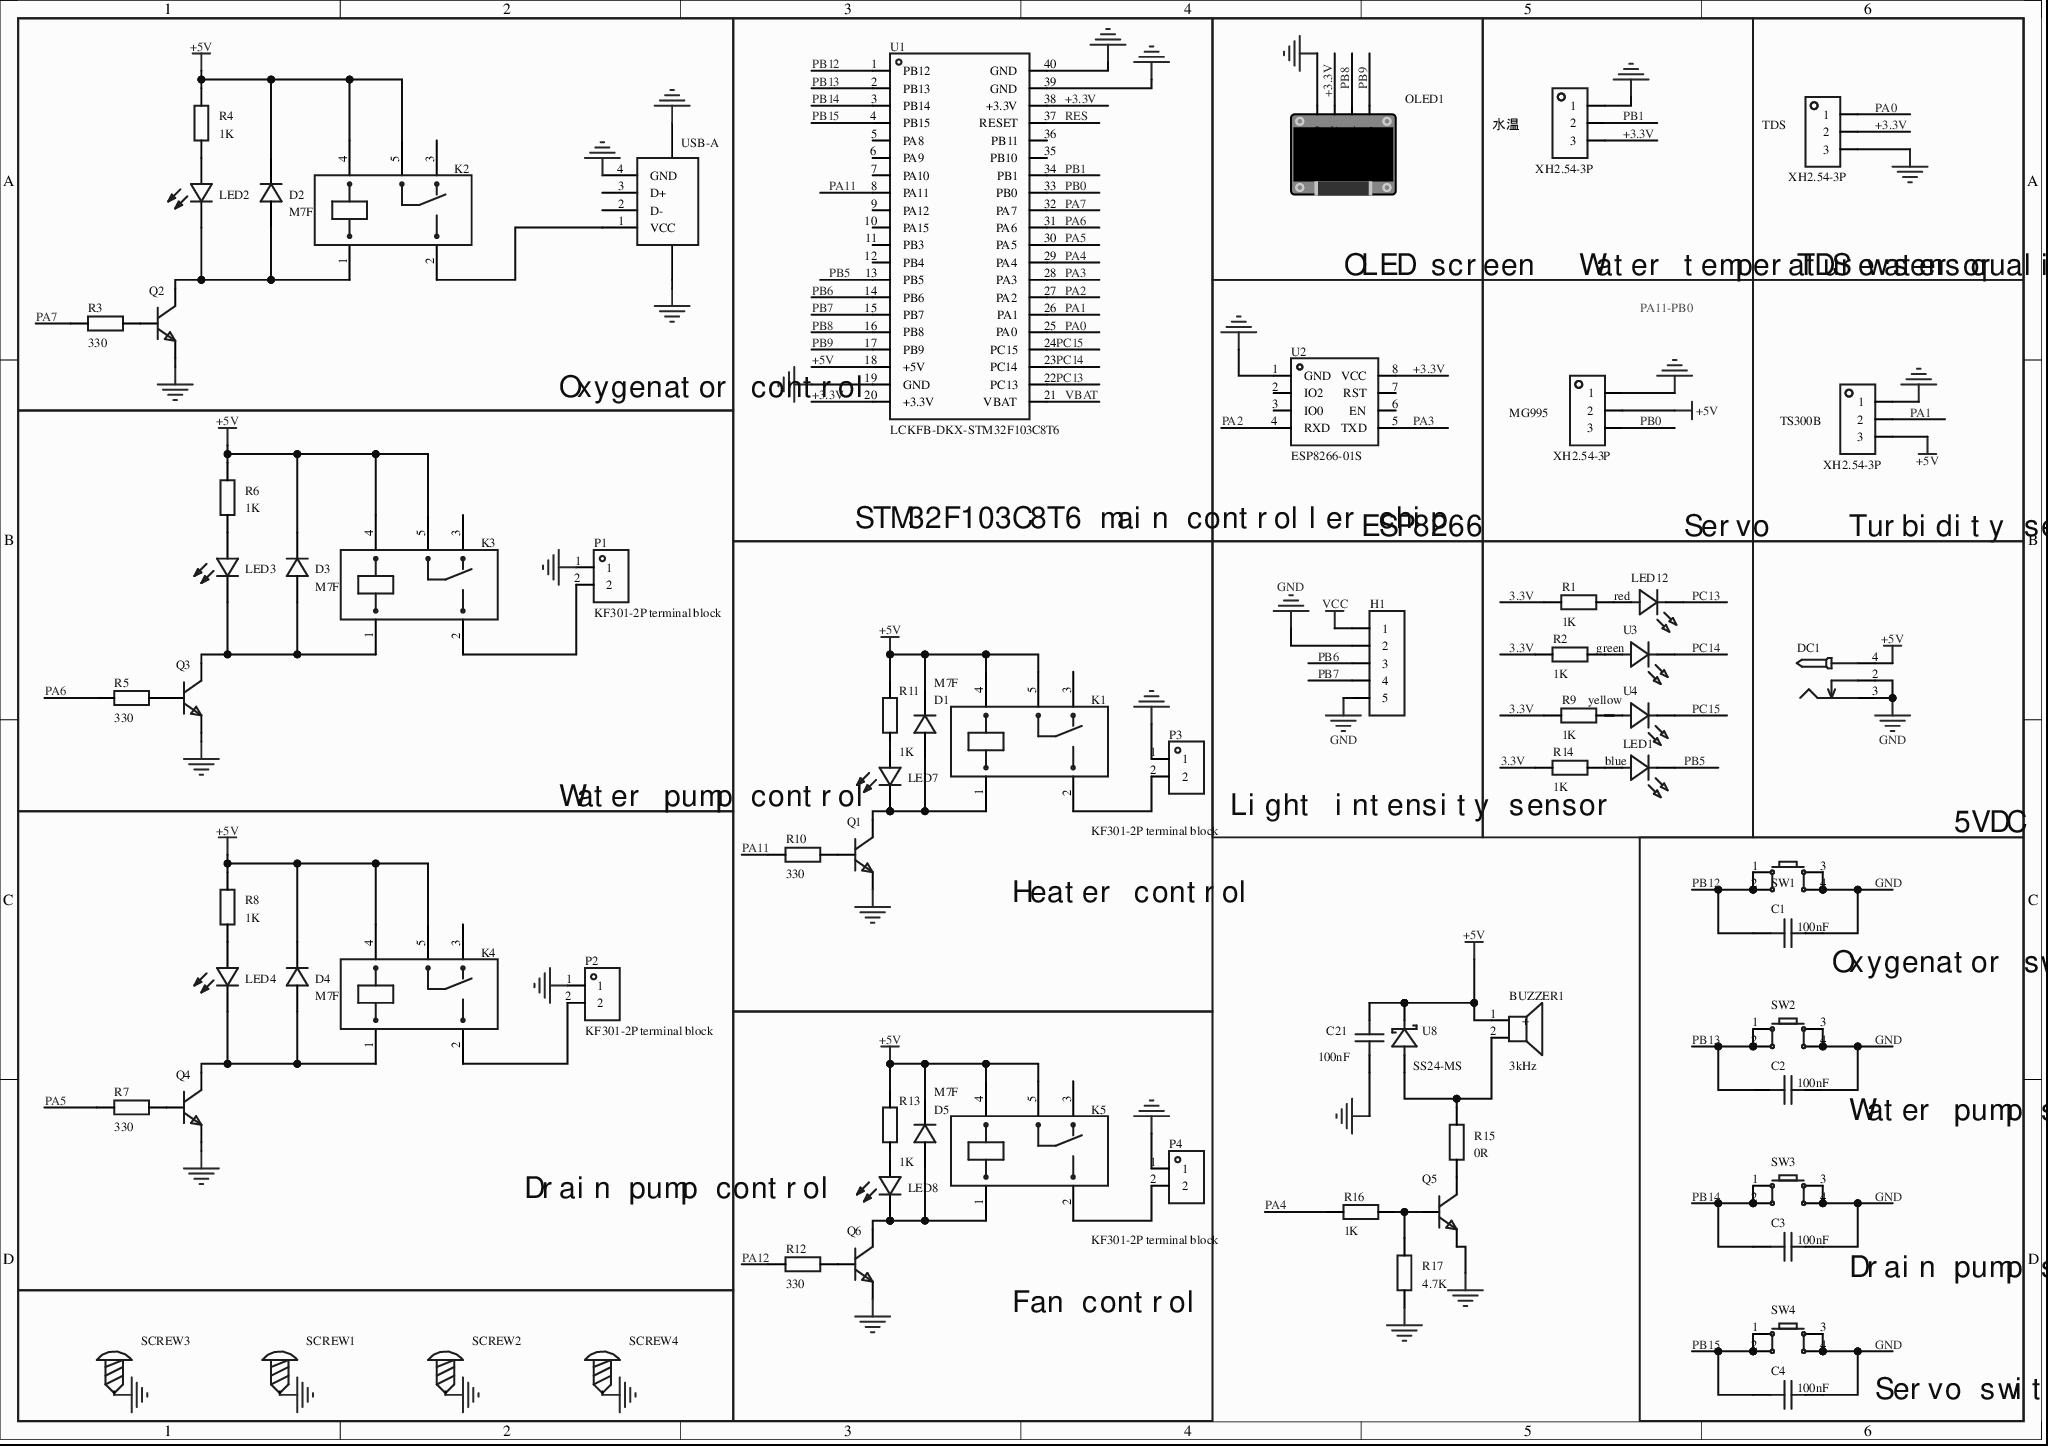
[diagram p0: MISC51727-3.schdoc]
# Altium project MISC51727.PrjPcb
1 sheet, 71 parts. Net scope: global (net labels, ports and power ports of the same name join across sheets).
Board file: MISC51727.pcbdoc

## Sheet MISC51727-3.schdoc
size 297 x 209 mm; Version: V1.0; @Project Name: MISC51727; @Page Count: 1; @Update Date: 2026-05-01; @Create Date: 2026-05-01; @Schematic Name: MISC51727; @Page No: 1; @Create Time: 10:53:21; @Update Time: 20:05:00; @Board Name: MISC51727

### Parts
BUZZER1  3kHz  [BUZ-TH_BD9.6-P5.00-D0.7-FD]
C1  100nF  [C0603]
C2  100nF  [C0603]
C3  100nF  [C0603]
C4  100nF  [C0603]
C21  100nF  [C0603]
D1  M7F  [SMAF_L3.5-W2.6-LS4.7-RD]
D2  M7F  [SMAF_L3.5-W2.6-LS4.7-RD]
D3  M7F  [SMAF_L3.5-W2.6-LS4.7-RD]
D4  M7F  [SMAF_L3.5-W2.6-LS4.7-RD]
D5  M7F  [SMAF_L3.5-W2.6-LS4.7-RD]
DC1  (no value)  [DC-2.0]
H1  (no value)  [HDR-TH_5P-P2.54-V-F]
K1  SRD-DC5V-SL-C  [RELAY-TH_SRD-DCXXV-SL-C]  (value not drawn)
K2  SRD-DC5V-SL-C  [RELAY-TH_SRD-DCXXV-SL-C]  (value not drawn)
K3  SRD-DC5V-SL-C  [RELAY-TH_SRD-DCXXV-SL-C]  (value not drawn)
K4  SRD-DC5V-SL-C  [RELAY-TH_SRD-DCXXV-SL-C]  (value not drawn)
K5  SRD-DC5V-SL-C  [RELAY-TH_SRD-DCXXV-SL-C]  (value not drawn)
LED1  blue  [LED-TH_BD5.9-P2.54-RD_BLUE]
LED2  MS-PTV1608NWAF-B02  [LED0603-RD]  (value not drawn)
LED3  MS-PTV1608NWAF-B02  [LED0603-RD]  (value not drawn)
LED4  MS-PTV1608NWAF-B02  [LED0603-RD]  (value not drawn)
LED7  MS-PTV1608NWAF-B02  [LED0603-RD]  (value not drawn)
LED8  MS-PTV1608NWAF-B02  [LED0603-RD]  (value not drawn)
LED12  red  [LED-TH_BD5.9-P2.54-RD_RED]
MG995  (no value)  [XH2.54-3P]
OLED1  (no value)  [0.96OLED_4P]
P1  KF301-2P terminal block  [CONN-TH_XY301V-A-5.0-2P]
P2  KF301-2P terminal block  [CONN-TH_XY301V-A-5.0-2P]
P3  KF301-2P terminal block  [CONN-TH_XY301V-A-5.0-2P]
P4  KF301-2P terminal block  [CONN-TH_XY301V-A-5.0-2P]
Q1  (no value)  [S8050_SOT-23]
Q2  (no value)  [S8050_SOT-23]
Q3  (no value)  [S8050_SOT-23]
Q4  (no value)  [S8050_SOT-23]
Q5  (no value)  [S8050_SOT-23]
Q6  (no value)  [S8050_SOT-23]
R1  1K  [R0603]
R2  1K  [R0603]
R3  330  [R0603]
R4  1K  [R0603]
R5  330  [R0603]
R6  1K  [R0603]
R7  330  [R0603]
R8  1K  [R0603]
R9  1K  [R0603]
R10  330  [R0603]
R11  1K  [R0603]
R12  330  [R0603]
R13  1K  [R0603]
R14  1K  [R0603]
R15  0R  [R0603]
R16  1K  [R0603]
R17  4.7K  [R0603]
SCREW1  (no value)  [M3螺丝]
SCREW2  (no value)  [M3螺丝]
SCREW3  (no value)  [M3螺丝]
SCREW4  (no value)  [M3螺丝]
SW1  (no value)  [SW-SMD_4P-L6.0-W6.0-P4.50-LS9.0-2]
SW2  (no value)  [SW-SMD_4P-L6.0-W6.0-P4.50-LS9.0-2]
SW3  (no value)  [SW-SMD_4P-L6.0-W6.0-P4.50-LS9.0-2]
SW4  (no value)  [SW-SMD_4P-L6.0-W6.0-P4.50-LS9.0-2]
TDS  (no value)  [XH2.54-3P]
TS300B  (no value)  [XH2.54-3P]
U1  LCKFB-DKX-STM32F103C8T6  [CONN-TH_L53.3-W22.9_STM32F103C8T6-CARD]
U2  ESP8266-01S  [WIFIM-TH_ESP8266-01S]
U3  green  [LED-TH_BD5.9-P2.54-RD_GREEN]
U4  yellow  [LED-TH_BD5.9-P2.54-RD_YELLOW]
U8  SS24-MS  [SMA_L4.3-W2.6-LS5.1-RD]
USB-A  USB-AF  [USB-A-TH_USB-302-T]  (value not drawn)
水温  (no value)  [XH2.54-3P]

### Blocks framed on the sheet
Oxygenator control: D2 K2 LED2 Q2 R3 R4 USB-A
STM32F103C8T6 main controller chip: U1
OLED screen: OLED1
Water temperature sensor: 水温
TDS water quality sensor: TDS
ESP8266: U2
Servo: MG995
Turbidity sensor: TS300B
Water pump control: D3 K3 LED3 P1 Q3 R5 R6
Light intensity sensor: H1
5VDC: DC1 LED1 LED12 R1 R2 R9 R14 U3 U4
Drain pump control: D4 K4 LED4 P2 Q4 R7 R8
Fan control: D5 K5 LED8 P4 Q6 R12 R13

### Nets
VCC: H1.1 OLED1.2(VCC) R1.1 R2.1 R9.1 R14.1 TDS.2 U1.20(+3.3V) U1.38(+3.3V) U2.8(VCC) 水温.3  [also labelled +3.3V, 3.3V]
+5V: BUZZER1.1(+) C21.2 D1.1(C) D2.1(C) D3.1(C) D4.1(C) D5.1(C) DC1.4 K1.4 K1.5 K2.4 K2.5 K3.4 K3.5 K4.4 K4.5 K5.4 K5.5 MG995.2 R4.2 R6.2 R8.2 R11.2 R13.2 TS300B.3 U1.18(+5V) U8.1(C)
GND: C1.2 C2.2 C3.2 C4.2 C21.1 DC1.2 DC1.3 H1.2 H1.5 MG995.1 OLED1.1(GND) P1.1 P2.1 P3.1 P4.1 Q1.2 Q2.2 Q3.2 Q4.2 Q5.2 Q6.2 R17.2 SCREW1.1 SCREW2.1 SCREW3.1 SCREW4.1 SW1.3 SW1.4 SW2.3 SW2.4 SW3.3 SW3.4 SW4.3 SW4.4 TDS.3 TS300B.1 U1.19(GND) U1.39(GND) U1.40(GND) U2.1(GND) USB-A.4(GND) USB-A.5 USB-A.6 水温.1
PA0: TDS.1 U1.25(PA0)
PA1: TS300B.2 U1.26(PA1)
PA2: U1.27(PA2) U2.4(RXD)
PA3: U1.28(PA3) U2.5(TXD)
PA4: R16.2 U1.29(PA4)
PA5: R7.2 U1.30(PA5)
PA6: R5.2 U1.31(PA6)
PA7: R3.2 U1.32(PA7)
PA11: R10.2 U1.8(PA11)
PA12: R12.2
PB0: MG995.3 U1.33(PB0)
PB1: U1.34(PB1) 水温.2
PB5: LED1.1(K) U1.13(PB5)
PB6: H1.3 U1.14(PB6)
PB7: H1.4 U1.15(PB7)
PB8: OLED1.3(SCL) U1.16(PB8)
PB9: OLED1.4(SDA) U1.17(PB9)
PB12: C1.1 SW1.1 SW1.2 U1.1(PB12)
PB13: C2.1 SW2.1 SW2.2 U1.2(PB13)
PB14: C3.1 SW3.1 SW3.2 U1.3(PB14)
PB15: C4.1 SW4.1 SW4.2 U1.4(PB15)
PC13: LED12.1(K) U1.22(PC13)
PC14: U1.23(PC14) U3.1(K)
PC15: U1.24(PC15) U4.1(K)
RES: U1.37(RESET)
VBAT: U1.21(VBAT)
NetBUZZER1_2: BUZZER1.2 R15.2 U8.2(A)
NetD1_2: D1.2(A) K1.1 LED7.1(-) Q1.3
NetD2_2: D2.2(A) K2.1 LED2.1(-) Q2.3
NetD3_2: D3.2(A) K3.1 LED3.1(-) Q3.3
NetD4_2: D4.2(A) K4.1 LED4.1(-) Q4.3
NetD5_2: D5.2(A) K5.1 LED8.1(-) Q6.3
NetK1_2: K1.2 P3.2
NetK2_2: K2.2 USB-A.1(VCC)
NetK3_2: K3.2 P1.2
NetK4_2: K4.2 P2.2
NetK5_2: K5.2 P4.2
NetLED1_2: LED1.2(A) R14.2
NetLED2_2: LED2.2(+) R4.1
NetLED3_2: LED3.2(+) R6.1
NetLED4_2: LED4.2(+) R8.1
NetLED7_2: LED7.2(+) R11.1
NetLED8_2: LED8.2(+) R13.1
NetLED12_2: LED12.2(A) R1.2
NetQ1_1: Q1.1 R10.1
NetQ2_1: Q2.1 R3.1
NetQ3_1: Q3.1 R5.1
NetQ4_1: Q4.1 R7.1
NetQ5_1: Q5.1 R16.1 R17.1
NetQ5_3: Q5.3 R15.1
NetQ6_1: Q6.1 R12.1
NetR2_2: R2.2 U3.2(A)
NetR9_2: R9.2 U4.2(A)

Not connected (* = marked no-connect by the designer): K1 3*; K2 3*; K3 3*; K4 3*; K5 3*; U1 5(PA8) 6(PA9) 7(PA10) 9(PA12) 10(PA15) 11(PB3) 12(PB4) 35(PB10) 36(PB11); U2 2(IO2)* 3(IO0)* 6(EN)* 7(RST)*; USB-A 2(D-)* 3(D+)*

### Notes on the sheet
- PA11-PB0
- Heater control
- (near C1) Oxygenator switch
- Water pump switch
- Drain pump switch
- Servo switch

### Library data of the parts
BUZZER1 = HNB09A05: Drive method: Active (built-in driver circuit); Construction type: Electromagnetic; Rated voltage: -; Frequency: 3kHz; Sound pressure (SPL): 85dB;; Manufacturer: 华能; AddInBom: yes; ModelId: 13273335caac486e928bafb4d9fdf12d0819f05c4eef4c71ace90d822a990e87; ModelName: BUZ-TH_D9.0-H5.5-P5.0; ModelTransform: 354.33,354.33,0,90,0,0,0,0,-177.165; Voltage - Supply: 3V~7V; Symbol: HNB09A05; Device: HNB09A05; LCSC Part Name: HNB09A05; SupplierPart: C96493; ManufacturerPart: HNB09A05; Supplier Footprint: 插件,D=9mm; JLCPCB Part Class: Extended Part; Datasheet: https://item.szlcsc.com/datasheet/HNB09A05/97698.html; Supplier: LCSC; ConvertToPcb: yes; FootprintName: BUZ-TH_BD9.6-P5.00-D0.7-FD; Driver Circuitry: Active (built-in driver circuit); Technology: Electromagnetic; Voltage Rating: -; Value: 3kHz; Current Consumption: -; Sound Pressure Level(SPL): 85dB; Diameter(φD): 9mm; Length: -; Width: -; Height: 5.7mm; Operating Temperature: -
C1-C4 = CC0603KRX7R5BB104: Capacitance: 100nF; Tolerance: ±10%; Rated voltage: 6.3V; Dielectric (temp. coefficient): X7R;; Manufacturer: YAGEO(国巨); AddInBom: yes; ModelId: ac125912035d415993ca9572d50418b1; ModelName: C0603_L1.6-W0.8-H0.8; ModelTransform: 62.992,31.496,0,0,0,0,0,0,0; Symbol: CC0603KRX7R5BB104; Device: CC0603KRX7R5BB104; LCSC Part Name: 100nF ±10% 6.3V; SupplierPart: C5445386; ManufacturerPart: CC0603KRX7R5BB104; Supplier Footprint: 0603; Datasheet: https://atta.szlcsc.com/upload/public/pdf/source/20230424/E18B5086BA02F13791E1DFCA214F4995.pdf; Supplier: LCSC; ConvertToPcb: yes; FootprintName: C0603; Value: 100nF; Voltage Rated: 6.3V; Temperature Coefficient: X7R
C21 = CAP_0603: Symbol: CapAcitance; ConvertToPcb: yes; ModelId: ac125912035d415993ca9572d50418b1; ModelName: C0603_L1.6-W0.8-H0.8; ModelTransform: 62.992,31.496,0,0,0,0,0,0,0; Device: CAP_0603; AddInBom: yes; Supplier Footprint: 0603; FootprintName: C0603; Value: 100nF
D1 D5 = M7F_C22368801: Forward voltage drop (Vf): 1.1V@1A; DC reverse withstand voltage (Vr): 1kV; Rectifier current: 1A;; Manufacturer: Wild Goose(威谷); 3D Model: 4caf566195a049cf809ac17c4d641932; 3D Model Transform: 183.0705,102.362,0,0,0,0,0,0,0; Reverse Leakage Current (Ir): 5uA@1kV; Non-Repetitive Peak Forward Surge Current: 30A; AddInBom: yes; ModelName: SMAF_L3.5-W2.6-LS4.7-RD-1; Symbol: M7F_C22368801; Device: M7F_C22368801; LCSC Part Name: M7F; Supplier Part: C22368801; Manufacturer Part: M7F; Supplier Footprint: SMAF; JLCPCB Part Class: Extended library; Datasheet: https://item.szlcsc.com/datasheet/M7F/23847113.html; Supplier: LCSC; Voltage - Forward(Vf@If): 1.1V@1A; Voltage - DC Reverse(Vr): 1kV; Current - Rectified: 1A; ConvertToPcb: yes; FootprintName: SMAF_L3.5-W2.6-LS4.7-RD
D2-D4 = M7F_C22368801: Forward voltage drop (Vf): 1.1V@1A; DC reverse withstand voltage (Vr): 1kV; Rectifier current: 1A;; Manufacturer: Wild Goose(威谷); AddInBom: yes; ModelId: 4caf566195a049cf809ac17c4d641932; ModelName: SMAF_L3.5-W2.6-LS4.7-RD-1; ModelTransform: 183.0705,102.362,0,0,0,0,0,0,0; Reverse Leakage Current (Ir): 5uA@1kV; Non-Repetitive Peak Forward Surge Current: 30A; Symbol: M7F_C22368801; Device: M7F_C22368801; LCSC Part Name: M7F; SupplierPart: C22368801; ManufacturerPart: M7F; Supplier Footprint: SMAF; JLCPCB Part Class: Extended library; Datasheet: https://item.szlcsc.com/datasheet/M7F/23847113.html; Supplier: LCSC; ConvertToPcb: yes; FootprintName: SMAF_L3.5-W2.6-LS4.7-RD; Voltage - Forward(Vf@If): 1.1V@1A; Voltage - DC Reverse(Vr): 1kV; Current - Rectified: 1A
DC1 = DC-005_2.0: Symbol: DC power jack; ConvertToPcb: yes; ModelId: f5f20b8a2308479b936ba3c2698865bb0819f05c4eef4c71ace90d822a990e87; ModelName: DC-IN-TH_DC-5520-1; ModelTransform: 372.05,551.18,582.68,90,0,0,137.8,0,-149.61; Device: DC-005_2.0; AddInBom: yes; Supplier Footprint: 插件; FootprintName: DC-2.0
H1 = HDR-F_2.54_1x5P: Symbol: Header-Female-2.54_1x5; ConvertToPcb: yes; ModelId: f49cb6116a3d45e5a64915bf3e00773f0819f05c4eef4c71ace90d822a990e87; ModelTransform: 519.684,98.464,0,0,0,0,0,0,-124.016; Device: HDR-F_2.54_1x5P; AddInBom: yes; SupplierPart: C50950; Supplier Footprint: 插件; FootprintName: HDR-TH_5P-P2.54-V-F; ModelName: HDR-TH_5P-P2.54-V-F
K1 K5 = SRD-DC5V-SL-C: Contact form: -;; 3D Model: d0eda9b8bf8746d18ae810ab88dc78e7; 3D Model Transform: 755.904,622.4397,0,0,0,0,34.882,0,-118.11; AddInBom: yes; ModelName: RELAY-TH_L19.2-W15.6-H15.8; Symbol: SRD-DC5V-SL-C; Device: SRD-DC5V-SL-C; LCSC Part Name: SRD-DC5V-SL-C; Supplier Part: C688865; Manufacturer Part: SRD-DC5V-SL-C; Supplier Footprint: 插件; JLCPCB Part Class: Extended library; Supplier: LCSC; Contact Form: -; Coil Type: -; ConvertToPcb: yes; FootprintName: RELAY-TH_SRD-DCXXV-SL-C
K2-K4 = SRD-DC5V-SL-C: Contact form: -;; AddInBom: yes; ModelId: d0eda9b8bf8746d18ae810ab88dc78e7; ModelName: RELAY-TH_L19.2-W15.6-H15.8; ModelTransform: 755.904,622.4397,0,0,0,0,34.882,0,-118.11; Symbol: SRD-DC5V-SL-C; Device: SRD-DC5V-SL-C; LCSC Part Name: SRD-DC5V-SL-C; SupplierPart: C688865; ManufacturerPart: SRD-DC5V-SL-C; Supplier Footprint: 插件; JLCPCB Part Class: Extended library; Supplier: LCSC; ConvertToPcb: yes; FootprintName: RELAY-TH_SRD-DCXXV-SL-C; Contact Form: -; Coil Type: -
LED1 = XL-502UBD: Lamp holder type: 5mm round lamp holder; Emitting color: Blue; Forward voltage drop (Vf): 3.4V; Power: 70mW; Forward current: 20mA; Wavelength: 460nm~470nm; Diode configuration: -; Lens color: Blue lens; Color temperature: -; Luminous intensity: 3cd; Viewing angle: 25°; Tape and reel: -; Operating temperature: -20℃~+85℃;; Manufacturer: XINGLIGHT(成兴光); AddInBom: yes; ModelId: fdce5b7de93842d7bd47dcb717270b810819f05c4eef4c71ace90d822a990e87; ModelTransform: 211.96686,228.01584,0,0,0,0,7.874,0,-137.795; Peak Wavelength: 465nm; Symbol: XL-502UBD; Device: XL-502UBD; Manufacturer Part: blue; LCSC Part Name: 5mm圆形灯头 蓝色; SupplierPart: C2895496; Supplier Footprint: 插件,D=5mm; JLCPCB Part Class: Extended Part; Datasheet: https://item.szlcsc.com/datasheet/XL-502UBD/3136211.html; Supplier: LCSC; ConvertToPcb: yes; FootprintName: LED-TH_BD5.9-P2.54-RD_BLUE; ModelName: LED-TH_BD5.9-P2.54-RD_BLUE; Lamp Holder Type: 5mm round lamp holder; Illumination Color: Blue; Voltage - Forward(Vf): 3.4V; Power(Watts): 70mW; Forward Current: 20mA; Wavelength - Dominant: 460nm~470nm; Diode Configuration: -; Lens Color: Blue lens; Color Temperature: -; Luminous Intensity: 3cd; Viewing Angle: 25°; Mounting Style: -; Operating Temperature: -20℃~+85℃
LED2-LED4 = MS-PTV1608NWAF-B02: AddInBom: yes; ModelId: 1f0d29a91be547639d425604e9b96ebb; ModelTransform: 63.7794,32.283,0,0,0,0,0,0,0; Symbol: MS-PTV1608NWAF-B02; Device: MS-PTV1608NWAF-B02; LCSC Part Name: MS-PTV1608NWAF-B02; SupplierPart: C9900092855; ManufacturerPart: MS-PTV1608NWAF-B02; Supplier Footprint: LED0603; JLCPCB Part Class: Extended library; Supplier: LCSC; ConvertToPcb: yes; FootprintName: LED0603-RD; ModelName: LED0603-RD
LED7 LED8 = MS-PTV1608NWAF-B02: 3D Model: 1f0d29a91be547639d425604e9b96ebb; 3D Model Transform: 63.7794,32.283,0,0,0,0,0,0,0; AddInBom: yes; Symbol: MS-PTV1608NWAF-B02; Device: MS-PTV1608NWAF-B02; LCSC Part Name: MS-PTV1608NWAF-B02; Supplier Part: C9900092855; Manufacturer Part: MS-PTV1608NWAF-B02; Supplier Footprint: LED0603; JLCPCB Part Class: Extended library; Supplier: LCSC; ConvertToPcb: yes; FootprintName: LED0603-RD; ModelName: LED0603-RD
LED12 = XL-502SURD: Lamp holder type: 5mm round lamp holder; Emitting color: Red; Forward voltage drop (Vf): 2.4V; Power: 70mW; Forward current: 20mA; Wavelength: 615nm~625nm; Diode configuration: -; Lens color: Red lens; Color temperature: -; Luminous intensity: 300mcd; Viewing angle: 35°; Tape and reel: -; Operating temperature: -25℃~+85℃;; Manufacturer: XINGLIGHT(成兴光); AddInBom: yes; ModelId: fe9cea1bdf7642cd8d9a5077ed0e2b580819f05c4eef4c71ace90d822a990e87; ModelTransform: 211.96686,228.01584,0,0,0,0,7.874,0,-137.795; Peak Wavelength: 654nm; Symbol: XL-502SURD; Device: XL-502SURD; Manufacturer Part: red; LCSC Part Name: 5mm圆形灯头 红色; SupplierPart: C2895492; Supplier Footprint: 插件,D=5mm; JLCPCB Part Class: Extended Part; Datasheet: https://item.szlcsc.com/datasheet/XL-502SURD/3136207.html; Supplier: LCSC; ConvertToPcb: yes; FootprintName: LED-TH_BD5.9-P2.54-RD_RED; ModelName: LED-TH_BD5.9-P2.54-RD_RED; Lamp Holder Type: 5mm round lamp holder; Illumination Color: Red; Voltage - Forward(Vf): 2.4V; Power(Watts): 70mW; Forward Current: 20mA; Wavelength - Dominant: 615nm~625nm; Diode Configuration: -; Lens Color: Red lens; Color Temperature: -; Luminous Intensity: 300mcd; Viewing Angle: 35°; Mounting Style: -; Operating Temperature: -25℃~+85℃
MG995 TDS TS300B 水温 = 弯针座3P: Device: Right-angle header 3P; AddInBom: yes; ModelId: 964060380ab84c59b2a38cefb7706dab0819f05c4eef4c71ace90d822a990e87; ModelName: CONN-TH_3P-P2.50_WAFER-XH2.54-3PWZ; ModelTransform: 322.82,246.39000000000001,299.92,180,0,0,0,118.11,-102.36; ConvertToPcb: yes; SymbolName: Right-angle header 3P; FootprintName: XH2.54-3P
OLED1 = 0.96OLED模块_4P: Device: 0.96OLED module_4P; ConvertToPcb: yes; ModelId: 79c000fdb68d45a296c2e9bedf4f9055; ModelTransform: 1393.69792,1318.895,0,0,0,0,0,-560.079,-137.795; AddInBom: yes; SymbolName: 0.96OLED module_4P; FootprintName: 0.96OLED_4P; Supplier Footprint: 插件; ModelName: 0.96OLED_4P
P1 P2 = KF301-2P接线端子: AddInBom: yes; ModelId: ef7ead88b0f2448d904975b26718870f; ModelTransform: 417.322,299.212,0,0,0,0,11.811,-7.835,-157.48; Symbol: KF301-2P terminal block; Device: KF301-2P terminal block; LCSC Part Name: KF301-2P接线端子; SupplierPart: C9900016950; ManufacturerPart: KF301-2P接线端子; Supplier Footprint: CK301-2P; JLCPCB Part Class: Extended library; Supplier: LCSC; ConvertToPcb: yes; FootprintName: CONN-TH_XY301V-A-5.0-2P; ModelName: CONN-TH_XY301V-A-5.0-2P
P3 P4 = KF301-2P接线端子: 3D Model: ef7ead88b0f2448d904975b26718870f; 3D Model Transform: 417.322,299.212,0,0,0,0,11.811,-7.835,-157.48; AddInBom: yes; Symbol: KF301-2P terminal block; Device: KF301-2P terminal block; LCSC Part Name: KF301-2P接线端子; Supplier Part: C9900016950; Manufacturer Part: KF301-2P接线端子; Supplier Footprint: CK301-2P; JLCPCB Part Class: Extended library; Supplier: LCSC; ConvertToPcb: yes; FootprintName: CONN-TH_XY301V-A-5.0-2P; ModelName: CONN-TH_XY301V-A-5.0-2P
Q1 Q6 = S8050_SOT_NPN: Symbol: NPN; 3D Model: c62791f0466c4ae2a892c056b845b0ca; 3D Model Transform: 98.6,114.12,41.29,180,0,0,0,0,-3; ConvertToPcb: yes; ModelName: SOT-23-3P_L2.9-W1.3-H1.0-LS2.4-P0.95; Device: S8050_SOT_NPN; Supplier Footprint: SOT-23; AddInBom: yes; FootprintName: S8050_SOT-23
Q2-Q4 = S8050_SOT_NPN: ConvertToPcb: yes; SymbolName: NPN; ModelId: c62791f0466c4ae2a892c056b845b0ca; ModelName: SOT-23-3P_L2.9-W1.3-H1.0-LS2.4-P0.95; ModelTransform: 98.6,114.12,41.29,180,0,0,0,0,-3; Device: S8050_SOT_NPN; AddInBom: yes; Supplier Footprint: SOT-23; FootprintName: S8050_SOT-23
Q5 = S8050_SOT_NPN: Symbol: NPN; ConvertToPcb: yes; ModelId: c62791f0466c4ae2a892c056b845b0ca; ModelName: SOT-23-3P_L2.9-W1.3-H1.0-LS2.4-P0.95; ModelTransform: 98.6,114.12,41.29,180,0,0,0,0,-3; Device: S8050_SOT_NPN; AddInBom: yes; Supplier Footprint: SOT-23; FootprintName: S8050_SOT-23
R1 R2 R9-R14 = Res_0603: Symbol: Resistor; 3D Model: fc143cca1e79419f9cd78b61e9279f08; 3D Model Transform: 31.8897,63.7794,0,90,0,0,0,0,0; ConvertToPcb: yes; Device: Res_0603; Supplier Footprint: 0603; AddInBom: yes; FootprintName: R0603; ModelName: R0603
  R1 R2 R9 R11 R13 R14: Value: 1K
  R10 R12: Value: 330
R3-R8 = Res_0603: ConvertToPcb: yes; SymbolName: Resistor; ModelId: fc143cca1e79419f9cd78b61e9279f08; ModelTransform: 31.8897,63.7794,0,90,0,0,0,0,0; Device: Res_0603; AddInBom: yes; Supplier Footprint: 0603; FootprintName: R0603; ModelName: R0603
  R3 R5 R7: Value: 330
  R4 R6 R8: Value: 1K
R15-R17 = Res_0603: Symbol: Resistor; ConvertToPcb: yes; ModelId: fc143cca1e79419f9cd78b61e9279f08; ModelTransform: 31.8897,63.7794,0,90,0,0,0,0,0; Device: Res_0603; AddInBom: yes; Supplier Footprint: 0603; FootprintName: R0603; ModelName: R0603
  R15: Value: 0R
  R16: Value: 1K
  R17: Value: 4.7K
SCREW1-SCREW4 = M3螺丝: Device: M3 screw; ConvertToPcb: yes; SymbolName: Screw hole; AddInBom: yes; Supplier Footprint: 插件; FootprintName: M3 screw
SW1-SW4 = Key_SMD_6x6x6.5: Symbol: Tactile switch; ConvertToPcb: yes; ModelId: fbf4ceca6c4742d48614ab6a891ef981; ModelName: SW-SMD_4P-L6.0-W6.0-P4.50-LS11.0; ModelTransform: 330.708,251.968,0,0,0,0,0,-0.005,0; Device: Key_SMD_6x6x6.5; AddInBom: yes; Supplier Footprint: SMD; FootprintName: SW-SMD_4P-L6.0-W6.0-P4.50-LS9.0-2
U1 = LCKFB-DKX-STM32F103C8T6: Manufacturer: 立创开发板; AddInBom: yes; ModelId: 12c257eccf3b4e5baa9346e6693d8ea4; Symbol: LCKFB-DKX-STM32F103C8T6; Device: LCKFB-DKX-STM32F103C8T6; LCSC Part Name: 立创·地阔星-STM32F103C8T6开发板; SupplierPart: C22396880; ManufacturerPart: LCKFB-DKX-STM32F103C8T6; Supplier Footprint: -; JLCPCB Part Class: Extended library; Datasheet: https://item.szlcsc.com/datasheet/LCKFB-DKX-STM32F103C8T6/24005615.html; Supplier: LCSC; ConvertToPcb: yes; FootprintName: CONN-TH_L53.3-W22.9_STM32F103C8T6-CARD; ModelName: CONN-TH_L53.3-W22.9_STM32F103C8T6-CARD
U2 = ESP8266-01S: AddInBom: yes; ModelId: 7671a3a19d0d4245ae5d5806b59f4d51; ModelTransform: 566.928,972.439,0,0,0,0,0,378.464,-118.11; Symbol: ESP8266-01S; Device: ESP8266-01S; LCSC Part Name: ESP8266-01S; SupplierPart: C9900150497; ManufacturerPart: ESP8266-01S; Supplier Footprint: TH-8P; JLCPCB Part Class: Extended library; Supplier: LCSC; ConvertToPcb: yes; FootprintName: WIFIM-TH_ESP8266-01S; ModelName: WIFIM-TH_ESP8266-01S
U3 = XL-502UGD: Lamp holder type: 5mm round lamp holder; Emitting color: Emerald green; Forward voltage drop (Vf): 3V; Power: 70mW; Forward current: 20mA; Wavelength: 520nm~530nm; Diode configuration: -; Lens color: Green lens; Color temperature: -; Luminous intensity: 12cd; Viewing angle: 25°; Tape and reel: -; Operating temperature: -25℃~+85℃;; Manufacturer: XINGLIGHT(成兴光); AddInBom: yes; ModelId: 0ecbca0d139a466b8fc3aef618bbaa4e0819f05c4eef4c71ace90d822a990e87; ModelTransform: 211.96686,228.01584,0,0,0,0,7.874,0,-216.535; Peak Wavelength: 520nm; Symbol: XL-502UGD; Device: XL-502UGD; Manufacturer Part: green; LCSC Part Name: 绿发翠绿短脚; SupplierPart: C2895548; Supplier Footprint: 插件,D=5mm; JLCPCB Part Class: Extended Part; Datasheet: https://item.szlcsc.com/datasheet/XL-502UGD/3136213.html; Supplier: LCSC; ConvertToPcb: yes; FootprintName: LED-TH_BD5.9-P2.54-RD_GREEN; ModelName: LED-TH_BD5.9-P2.54-RD_GREEN; Lamp Holder Type: 5mm round lamp holder; Illumination Color: Emerald green; Voltage - Forward(Vf): 3V; Power(Watts): 70mW; Forward Current: 20mA; Wavelength - Dominant: 520nm~530nm; Diode Configuration: -; Lens Color: Green lens; Color Temperature: -; Luminous Intensity: 12cd; Viewing Angle: 25°; Mounting Style: -; Operating Temperature: -25℃~+85℃
U4 = XL-502UYD: Lamp holder type: 5mm round lamp holder; Emitting color: Yellow; Forward voltage drop (Vf): 2.2V; Power: 50mW; Forward current: 20mA; Wavelength: 585nm~595nm; Diode configuration: -; Lens color: Yellow lens; Color temperature: -; Luminous intensity: 1cd; Viewing angle: 25°; Tape and reel: -; Operating temperature: -20℃~+85℃;; Manufacturer: XINGLIGHT(成兴光); AddInBom: yes; ModelId: 60b947332da4492684d7623f83070ee30819f05c4eef4c71ace90d822a990e87; ModelTransform: 211.96686,228.01584,0,0,0,0,7.874,0,-137.795; Peak Wavelength: 588nm; Symbol: XL-502UYD; Device: XL-502UYD; Manufacturer Part: yellow; LCSC Part Name: 5mm圆形灯头 黄色; SupplierPart: C2895494; Supplier Footprint: 插件,D=5mm; JLCPCB Part Class: Extended Part; Datasheet: https://item.szlcsc.com/datasheet/XL-502UYD/3136209.html; Supplier: LCSC; ConvertToPcb: yes; FootprintName: LED-TH_BD5.9-P2.54-RD_YELLOW; ModelName: LED-TH_BD5.9-P2.54-RD_YELLOW; Lamp Holder Type: 5mm round lamp holder; Illumination Color: Yellow; Voltage - Forward(Vf): 2.2V; Power(Watts): 50mW; Forward Current: 20mA; Wavelength - Dominant: 585nm~595nm; Diode Configuration: -; Lens Color: Yellow lens; Color Temperature: -; Luminous Intensity: 1cd; Viewing Angle: 25°; Mounting Style: -; Operating Temperature: -20℃~+85℃
U8 = SS24-MS: Diode configuration: -; Forward voltage drop (Vf): 550mV@2A; DC reverse withstand voltage (Vr): 40V; Rectifier current: 2A;; Manufacturer: MSKSEMI(美森科); AddInBom: yes; ModelId: 1d20a911e9694ba6aaf6e9207164e4da; ModelTransform: 196.4563,102.362,0,0,0,0,0,0,0; Reverse Leakage Current (Ir): 500uA@40V; Operating Junction Temperature Range: -65℃~+125℃; Non-Repetitive Peak Forward Surge Current: 50A; Symbol: SS24-MS; Device: SS24-MS; LCSC Part Name: 电压:40V 电流:2A; SupplierPart: C2836395; ManufacturerPart: SS24-MS; Supplier Footprint: SMA(DO-214AC); JLCPCB Part Class: Extended library; Datasheet: https://item.szlcsc.com/datasheet/SS24-MS/3002240.html; Supplier: LCSC; ConvertToPcb: yes; FootprintName: SMA_L4.3-W2.6-LS5.1-RD; ModelName: SMA_L4.3-W2.6-LS5.1-RD; Diode Configuration: -; Voltage - Forward(Vf@If): 550mV@2A; Voltage - DC Reverse(Vr): 40V; Current - Rectified: 2A
USB-A = USB-AF: AddInBom: yes; ModelId: ea4ed751d3d54744b981ffceb9921ba8; ModelName: USB-A-TH_USB-A-F-90; ModelTransform: 578.11097,563.188,0,0,0,0,0.5,-207.856,-169.291; Symbol: USB-AF; Device: USB-AF; LCSC Part Name: USB-AF; SupplierPart: C9900021158; ManufacturerPart: USB-AF; Supplier Footprint: USB-A; JLCPCB Part Class: Extended library; Supplier: LCSC; ConvertToPcb: yes; FootprintName: USB-A-TH_USB-302-T